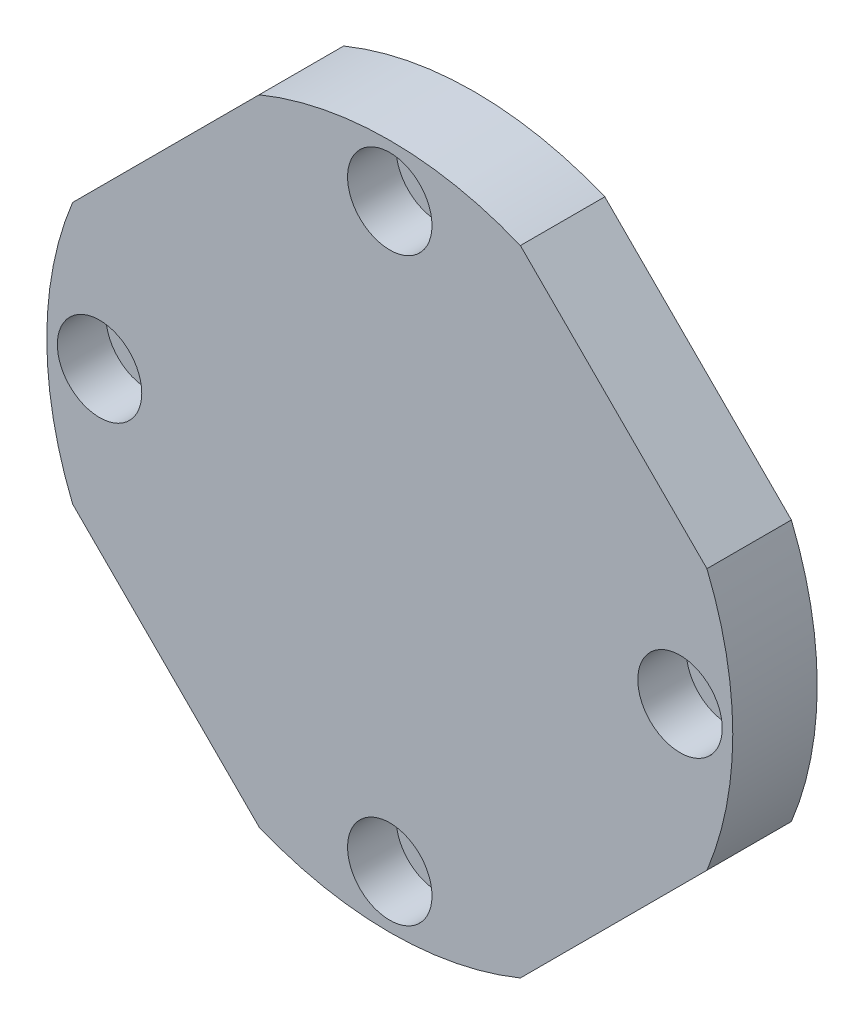
from build123d import *

# Parameters (mm, degrees)
BOSS_EXTRUDE1_DEPTH                                  = 8
HOLE_SIZE_PER_SOCKET_HEAD_CAP_SCREW_TYPE_D           = 4.5
HOLE_SIZE_PER_SOCKET_HEAD_CAP_SCREW_TYPE_CBORE_D     = 8
HOLE_SIZE_PER_SOCKET_HEAD_CAP_SCREW_TYPE_CBORE_DEPTH = 4.6


with BuildPart() as part:
    # Sketch1 → Boss-Extrude1 (new body)
    with BuildSketch(Plane.XY):
        with BuildLine():
            Line((-30.0520382, -12.374368671), (-12.374368671, -30.0520382))
            ThreePointArc((-12.374368671, -30.0520382), (0, -32.5), (12.374368671, -30.0520382))
            Line((12.374368671, -30.0520382), (30.0520382, -12.374368671))
            ThreePointArc((30.0520382, -12.374368671), (32.5, 0), (30.0520382, 12.374368671))
            Line((30.0520382, 12.374368671), (12.374368671, 30.0520382))
            ThreePointArc((12.374368671, 30.0520382), (0, 32.5), (-12.374368671, 30.0520382))
            Line((-12.374368671, 30.0520382), (-30.0520382, 12.374368671))
            ThreePointArc((-30.0520382, 12.374368671), (-32.5, 0), (-30.0520382, -12.374368671))
        make_face()
    extrude(amount=BOSS_EXTRUDE1_DEPTH)

    # Hole size per socket head cap screw type 1 (through all)
    with Locations(Plane.XY.offset(8)):
        with Locations((0, 27.5), (-27.5, 0), (0, -27.5), (27.5, 0)):
            CounterBoreHole(HOLE_SIZE_PER_SOCKET_HEAD_CAP_SCREW_TYPE_D / 2, HOLE_SIZE_PER_SOCKET_HEAD_CAP_SCREW_TYPE_CBORE_D / 2, HOLE_SIZE_PER_SOCKET_HEAD_CAP_SCREW_TYPE_CBORE_DEPTH)


solid = part.part
